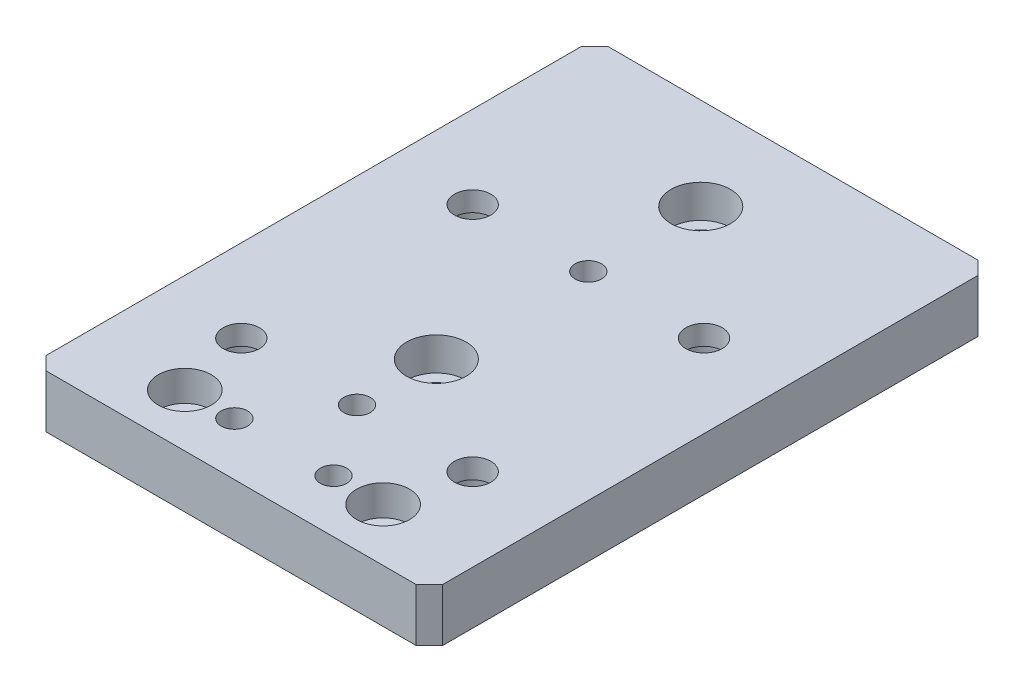
SolidWorks part; units mm, degrees
material "6061 合金"
ref_plane "前视" through (0, 0, 0) normal (0, 0, 1) x (1, 0, 0)
ref_plane "上视" through (0, 0, 0) normal (0, 1, 0) x (1, 0, 0)
ref_plane "右视" through (0, 0, 0) normal (1, 0, 0) x (0, 0, -1)
sketch "草图1" plane through (0, 0, 0) normal (0, 1, 0) x (1, 0, 0)
  line L1 (-30, -42.5) -> (30, -42.5)
  line L2 (-30, -42.5) -> (-30, 42.5)
  line L3 (-30, 42.5) -> (30, 42.5)
  line L4 (30, -42.5) -> (30, 42.5)
  line L5 (-30, -42.5) -> (30, 42.5) construction
  line L6 (-30, 42.5) -> (30, -42.5) construction
  point P0 (0, 0)
  dimension "D1" = 60
  dimension "D2" = 85
extrude "凸台-拉伸1" add sketch "草图1" along normal blind 8
hole_wizard "大小六角凹头盖螺钉柱孔1" positions "草图2" profile "草图3" counterbore size "M5" standard "AS" end condition through all
sketch "草图2" plane through (0, 0, 0) normal (0, -1, 0) x (-1, 0, 0)
  line L0 (0, 42.5) -> (0, -42.5) construction
  line L1 (-30, 42.5) -> (30, 42.5) construction
  line L2 (30, -42.5) -> (-30, -42.5) construction
  point P2 (17.5, -23.45)
  point P5 (-17.5, -23.45)
  point P8 (17.5, 11.55)
  point P11 (-17.5, 11.55)
  dimension "D1" = 35
  dimension "D2" = 19.05
  dimension "D3" = 35
sketch "草图3" plane through (-17.5, 0, 23.45) normal (1, 0, 0) x (0, 0, -1)
  line L0 (0, 0) -> (0, 8)
  line L1 (0, 8) -> (2.75, 8)
  line L3 (2.75, 8) -> (2.75, 5)
  line L4 (2.75, 5) -> (4.5, 5)
  line L5 (4.5, 5) -> (4.5, 0)
  line L7 (4.5, 0) -> (0, 0)
  line L11 (0, -6.35) -> (0, 107.95) construction
  dimension "通孔孔直径" = 5.5
  dimension "通孔孔深度" = 8
  dimension "柱形沉头孔直径" = 9
  dimension "柱形沉头孔深度" = 5
hole_wizard "大小六角凹头盖螺钉柱孔2" positions "草图7" profile "草图8" counterbore size "M5" standard "AS"
sketch "草图7" plane through (0, 8, 0) normal (0, 1, 0) x (1, 0, 0)
  line L1 (-30, -42.5) -> (30, -42.5) construction
  point P0 (0, 28.5545)
  point P3 (0, -11.4455)
  dimension "D1" = 31.0545
  dimension "D2" = 40
sketch "草图8" plane through (0, 8, -28.5545) normal (1, 0, 0) x (0, 0, 1)
  line L0 (0, 0) -> (0, 14.0524)
  line L1 (0, 14.0524) -> (2.75, 12.4)
  line L2 (2.75, 12.4) -> (2.75, 5)
  line L3 (2.75, 5) -> (4.5, 5)
  line L4 (4.5, 5) -> (4.5, 0)
  line L5 (4.5, 0) -> (0, 0)
  line L10 (0, 14.0524) -> (-2.75, 12.4) construction
  line L11 (0, -6.35) -> (0, 107.95) construction
  dimension "孔直径" = 5.5
  dimension "孔深度" = 12.4
  dimension "柱形沉头孔直径" = 9
  dimension "柱形沉头孔深度" = 5
  dimension "导头角度" = 118
hole_wizard "打孔尺寸(%根据)内六角圆柱头螺钉的类型1" positions "草图11" profile "草图12" counterbore size "M4" standard "GB" end condition through all
sketch "草图11" plane through (0, 8, 0) normal (0, 1, 0) x (1, 0, 0)
  line L0 (0, 0) -> (0, -42.5) construction
  line L1 (-30, -42.5) -> (30, -42.5) construction
  point P0 (-15, -34.5)
  point P3 (15, -34.5)
  dimension "D1" = 30
  dimension "D2" = 8
sketch "草图12" plane through (-15, 8, 34.5) normal (1, 0, 0) x (0, 0, 1)
  line L0 (0, 0) -> (0, 8)
  line L1 (0, 8) -> (2.25, 8)
  line L3 (2.25, 8) -> (2.25, 4.6)
  line L4 (2.25, 4.6) -> (4, 4.6)
  line L5 (4, 4.6) -> (4, 0)
  line L7 (4, 0) -> (0, 0)
  line L11 (0, -6.35) -> (0, 107.95) construction
  dimension "通孔孔直径" = 4.5
  dimension "通孔孔深度" = 8
  dimension "柱形沉头孔直径" = 8
  dimension "柱形沉头孔深度" = 4.6
hole_wizard "Ø4.0 (4) 直径孔1" positions "草图13" profile "草图14" hole size "Ø4.0" standard "ISO" end condition through all
sketch "草图13" plane through (0, 8, 0) normal (0, 1, 0) x (1, 0, 0)
  line L0 (0, 0) -> (0, -42.5) construction
  line L1 (-30, -42.5) -> (30, -42.5) construction
  line L2 (-30, -42.5) -> (30, -42.5) construction
  point P0 (-7.5, -34.5)
  point P2 (7.5, -34.5)
  point P12 (0, -23.45)
  point P15 (0, 11.55)
  dimension "D1" = 15
  dimension "D2" = 8
  dimension "D3" = 19.05
  dimension "D4" = 35
sketch "草图14" plane through (-7.5, 8, 34.5) normal (1, 0, 0) x (0, 0, 1)
  line L0 (0, 0) -> (0, 8)
  line L1 (0, 8) -> (2, 8)
  line L2 (2, 8) -> (2, 0)
  line L5 (2, 0) -> (0, 0)
  line L11 (0, -6.35) -> (0, 107.95) construction
  dimension "通孔孔直径" = 4
  dimension "通孔孔深度" = 8
chamfer "倒角1" distance 2 angle 45 4 edges at (-30, 4, -42.5) (30, 4, -42.5) (30, 4, 42.5) (-30, 4, 42.5)
